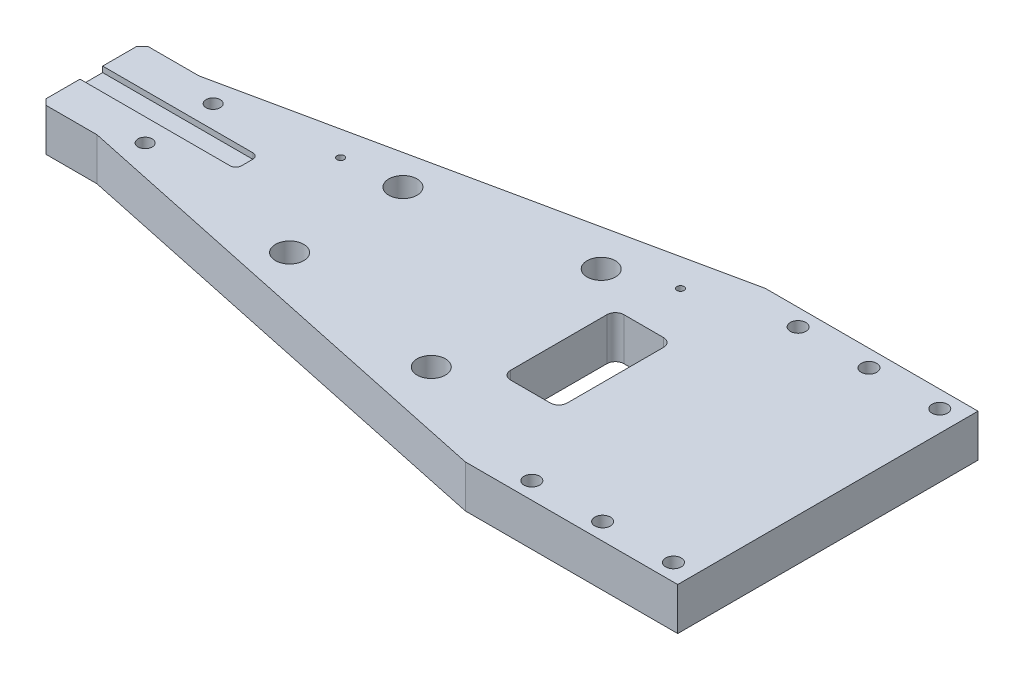
from build123d import *

# Parameters (mm, degrees)
SKETCH1_W                                            = 260
SKETCH1_H                                            = 106
BOSS_EXTRUDE1_DEPTH                                  = 7.5
CUT_EXTRUDE1_DEPTH                                   = 142.187818171
CUT_EXTRUDE2_DEPTH                                   = 2
M6_TAPPED_HOLE1_D                                    = 5
SKETCH9_W                                            = 20
SKETCH9_H                                            = 40
CUT_EXTRUDE4_DEPTH                                   = 142.187818171
FILLET5_R                                            = 3
HOLE_SIZE_PER_SOCKET_HEAD_CAP_SCREW_TYPE_D           = 5.5
HOLE_SIZE_PER_SOCKET_HEAD_CAP_SCREW_TYPE_CBORE_D     = 10
HOLE_SIZE_PER_SOCKET_HEAD_CAP_SCREW_TYPE_CBORE_DEPTH = 6
CHAMFER1_SIZE                                        = 2
M3_TAPPED_HOLE1_D                                    = 2.5
M3_TAPPED_HOLE1_DEPTH                                = 7.5
M3_TAPPED_HOLE1_TIP                                  = 0.751075774
F_10_0_10_DIAMETER_HOLE1_D                           = 10


with BuildPart() as part:
    # Sketch1 → Boss-Extrude1 (new, symmetric)
    with BuildSketch(Plane(origin=(0, 0, 0), x_dir=(1, 0, 0), z_dir=(0, 1, 0))):
        Rectangle(SKETCH1_W, SKETCH1_H)
    extrude(amount=BOSS_EXTRUDE1_DEPTH, both=True)

    # Sketch2 → Cut-Extrude1 (cut, through all)
    with BuildSketch(Plane(origin=(0, 7.5, 0), x_dir=(1, 0, 0), z_dir=(0, 1, 0))):
        Polygon((55, 53), (-130, 53), (-130, 18), (-110, 18), align=None)
        Polygon((-130, -18), (-130, -53), (55, -53), (-110, -18), align=None)
    extrude(amount=-CUT_EXTRUDE1_DEPTH, mode=Mode.SUBTRACT)

    # Sketch3 → Cut-Extrude2 (cut)
    with BuildSketch(Plane(origin=(0, 7.5, 0), x_dir=(1, 0, 0), z_dir=(0, 1, 0))):
        with BuildLine():
            Line((-130, 4), (-77, 4))
            ThreePointArc((-77, 4), (-75.585786438, 3.414213562), (-75, 2))
            Line((-75, 2), (-75, -2))
            ThreePointArc((-75, -2), (-75.585786438, -3.414213562), (-77, -4))
            Line((-77, -4), (-130, -4))
            Line((-130, -4), (-130, 4))
        make_face()
    extrude(amount=-CUT_EXTRUDE2_DEPTH, mode=Mode.SUBTRACT)

    # M6 Tapped Hole1 (through all)
    with Locations(Plane(origin=(0, 7.5, 0), x_dir=(1, 0, 0), z_dir=(0, 1, 0))):
        with Locations((-99, 12), (-99, -12)):
            Hole(M6_TAPPED_HOLE1_D / 2)

    # Sketch9 → Cut-Extrude4 (cut, through all)
    with BuildSketch(Plane(origin=(0, 7.5, 0), x_dir=(1, 0, 0), z_dir=(0, 1, 0))):
        with Locations((45, 0)):
            Rectangle(SKETCH9_W, SKETCH9_H)
    extrude(amount=-CUT_EXTRUDE4_DEPTH, mode=Mode.SUBTRACT)

    # Fillet5
    fillet5_edges = [part.edges().sort_by_distance(p)[0] for p in [
        (55, 0, -20),
        (55, 0, 20),
        (35, 0, 20),
        (35, 0, -20),
    ]]
    fillet(fillet5_edges, radius=FILLET5_R)

    # Hole size per socket head cap screw type1 (through all)
    with Locations(Plane(origin=(0, -7.5, 0), x_dir=(-1, 0, 0), z_dir=(0, -1, 0))):
        with Locations((-122.5, -47), (-97.5, -47), (-72.5, -47), (-72.5, 47), (-97.5, 47), (-122.5, 47)):
            CounterBoreHole(HOLE_SIZE_PER_SOCKET_HEAD_CAP_SCREW_TYPE_D / 2, HOLE_SIZE_PER_SOCKET_HEAD_CAP_SCREW_TYPE_CBORE_D / 2, HOLE_SIZE_PER_SOCKET_HEAD_CAP_SCREW_TYPE_CBORE_DEPTH)

    # Chamfer1
    chamfer1_edges = [part.edges().sort_by_distance(p)[0] for p in [
        (-130, 0, -18),
        (-130, 0, 18),
    ]]
    chamfer(chamfer1_edges, length=CHAMFER1_SIZE)

    # M3 Tapped Hole1
    with Locations(Plane(origin=(0, 7.5, 0), x_dir=(1, 0, 0), z_dir=(0, 1, 0))):
        with Locations((40, 38), (-60, 18)):
            Hole(M3_TAPPED_HOLE1_D / 2, depth=M3_TAPPED_HOLE1_DEPTH)
            with Locations((0, 0, -(M3_TAPPED_HOLE1_DEPTH + M3_TAPPED_HOLE1_TIP / 2))):  # 118° drill point
                Cone(0, M3_TAPPED_HOLE1_D / 2, M3_TAPPED_HOLE1_TIP, mode=Mode.SUBTRACT)

    # Ø10.0 (10) Diameter Hole1 (through all)
    with Locations(Plane(origin=(0, 7.5, 0), x_dir=(1, 0, 0), z_dir=(0, 1, 0))):
        with Locations((-40, 20), (-40, -20), (20, -30), (20, 30)):
            Hole(F_10_0_10_DIAMETER_HOLE1_D / 2)


solid = part.part
